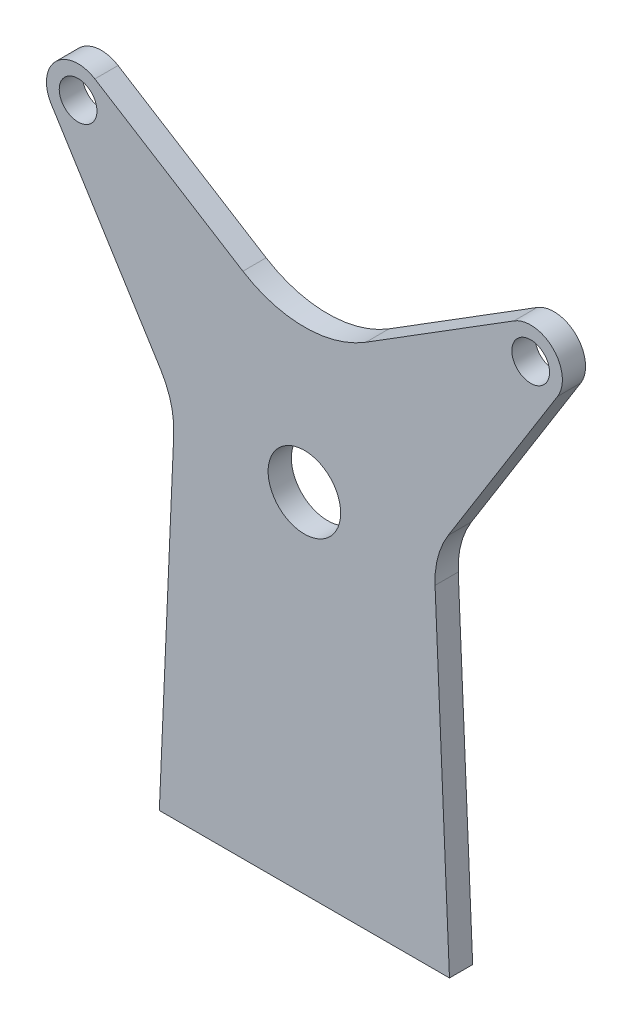
SolidWorks part; units mm, degrees
material "Q235B"
ref_plane "Front Plane" through (0, 0, 0) normal (0, 0, 1) x (1, 0, 0)
ref_plane "Top Plane" through (0, 0, 0) normal (0, 1, 0) x (1, 0, 0)
ref_plane "Right Plane" through (0, 0, 0) normal (1, 0, 0) x (0, 0, -1)
sketch "Sketch1" plane through (0, 0, 0) normal (0, 0, 1) x (1, 0, 0)
  line L0 (50, 0) -> (-50, 0)
  line L1 (-50, 0) -> (-45.0281, 114.7008)
  line L2 (-49.5586, 131.8976) -> (-87.2516, 192.219)
  line L3 (-72.219, 207.2516) -> (-21.1968, 175.3693)
  line L4 (0, 169.2913) -> (0, 0) construction
  line L5 (72.219, 207.2516) -> (21.1968, 175.3693)
  line L6 (49.5586, 131.8976) -> (87.2516, 192.219)
  line L7 (50, 0) -> (45.0281, 114.7008)
  line L8 (-78, 198) -> (19.893, 100.107) construction
  arc A0 (-45.0281, 114.7008) -> (-49.5586, 131.8976) centre (-75, 116) ccw
  arc A1 (-87.2516, 192.219) -> (-72.219, 207.2516) centre (-78, 198) cw
  arc A2 (-21.1968, 175.3693) -> (0, 169.2913) centre (0, 209.2913) ccw
  arc A3 (21.1968, 175.3693) -> (0, 169.2913) centre (0, 209.2913) cw
  arc A4 (87.2516, 192.219) -> (72.219, 207.2516) centre (78, 198) ccw
  arc A5 (45.0281, 114.7008) -> (49.5586, 131.8976) centre (75, 116) cw
  circle A6 centre (0, 120) radius 12.5
  circle A7 centre (78, 198) radius 6.5
  circle A9 centre (-78, 198) radius 6.5
  dimension "D1" = 100
  dimension "D3" = 30
  dimension "D4" = 40
  dimension "D10" = 25
  dimension "D11" = 13
  dimension "D2" = 150
  dimension "D5" = 156
  dimension "D6" = 198
  dimension "D7" = 26
  dimension "D8" = 64
  dimension "D9" = 116
extrude "Boss-Extrude1" add sketch "Sketch1" along normal mid plane 8
